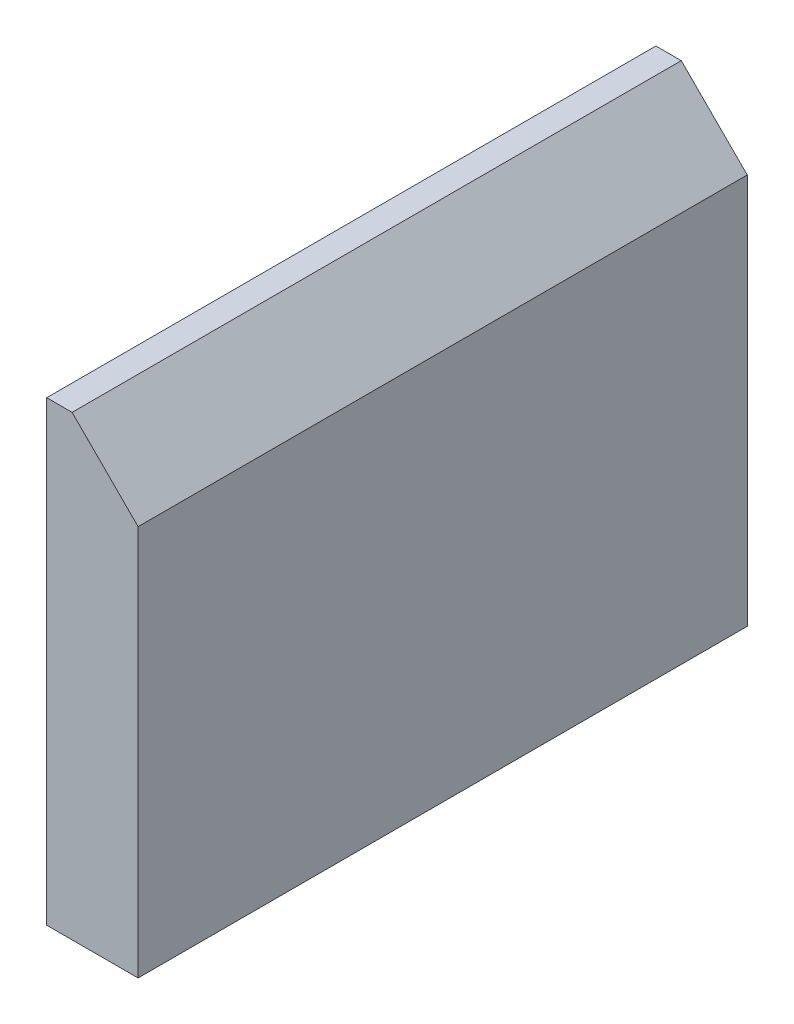
SolidWorks part; units mm, degrees
ref_plane "前视基准面" through (0, 0, 0) normal (0, 0, 1) x (1, 0, 0)
ref_plane "上视基准面" through (0, 0, 0) normal (0, 1, 0) x (1, 0, 0)
ref_plane "右视基准面" through (0, 0, 0) normal (1, 0, 0) x (0, 0, -1)
sketch "草图1" plane through (0, 0, 0) normal (0, 0, 1) x (1, 0, 0)
  line L0 (0, 9) -> (0, 0)
  line L1 (0, 0) -> (1.8, 0)
  line L2 (1.8, 0) -> (1.8, 7.7)
  line L3 (1.8, 7.7) -> (0.5, 9)
  line L4 (0.5, 9) -> (0, 9)
  dimension "D1" = 9
  dimension "D2" = 1.8
  dimension "D3" = 0.5
  dimension "D4" = 135
extrude "凸台-拉伸1" add sketch "草图1" along normal blind 12
